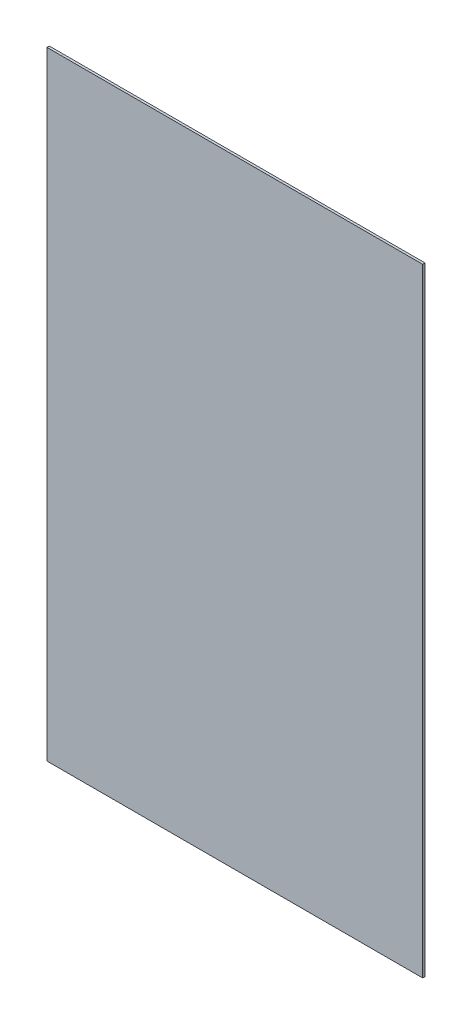
SolidWorks part; units mm, degrees
material "PMMA(有机玻璃)"
ref_plane "前视" through (0, 0, 0) normal (0, 0, 1) x (1, 0, 0)
ref_plane "上视" through (0, 0, 0) normal (0, 1, 0) x (1, 0, 0)
ref_plane "右视" through (0, 0, 0) normal (1, 0, 0) x (0, 0, -1)
sketch "草图1" plane through (0, 0, 0) normal (0, 0, 1) x (1, 0, 0)
  line L1 (-397, 653) -> (397, 653)
  line L2 (-397, 653) -> (-397, -653)
  line L3 (-397, -653) -> (397, -653)
  line L4 (397, 653) -> (397, -653)
  line L5 (-397, 653) -> (397, -653) construction
  line L6 (-397, -653) -> (397, 653) construction
  point P0 (0, 0)
  dimension "D1" = 1306
  dimension "D2" = 794
extrude "凸台-拉伸1" add sketch "草图1" along normal blind 5
hole_wizard "M5 间隙孔1" positions "草图3" profile "草图2" hole size "M5" standard "GB"
sketch "草图3" plane through (0, 0, 5) normal (0, 0, 1) x (1, 0, 0)
  line L0 (-427.5, 273) -> (-427.5, -273) construction
  line L1 (-427.5, -273) -> (427.5, -273) construction
  line L2 (0, 273) -> (0, -273) construction
  line L3 (427.5, 273) -> (-427.5, 273) construction
  line L5 (-427.5, 0) -> (427.5, 0) construction
  line L6 (427.5, -273) -> (427.5, 273) construction
  point P0 (-375, -261)
  point P46 (415.5, 250)
  point P48 (-415.5, 250)
  point P58 (-125, -261)
  point P59 (125, -261)
  point P61 (-125, 261)
  point P62 (125, 261)
  point P64 (-375, 261)
  point P88 (375, -261)
  point P89 (375, 261)
  point P108 (415.5, 0)
  point P109 (-415.5, 0)
  point P110 (415.5, -250)
  point P111 (-415.5, -250)
  dimension "D1" = 12
  dimension "D2" = 12
  dimension "D5" = 3
  dimension "D3" = 12
  dimension "D6" = 4
  dimension "D4" = 2
sketch "草图2" plane through (-375, -261, 5) normal (1, 0, 0) x (0, -1, 0)
  line L0 (0, 0) -> (0, 5)
  line L1 (0, 5) -> (2.75, 5)
  line L2 (2.75, 5) -> (2.75, 0)
  line L5 (2.75, 0) -> (0, 0)
  line L11 (0, -6.35) -> (0, 107.95) construction
  dimension "通孔孔直径" = 5.5
  dimension "通孔孔深度" = 5
